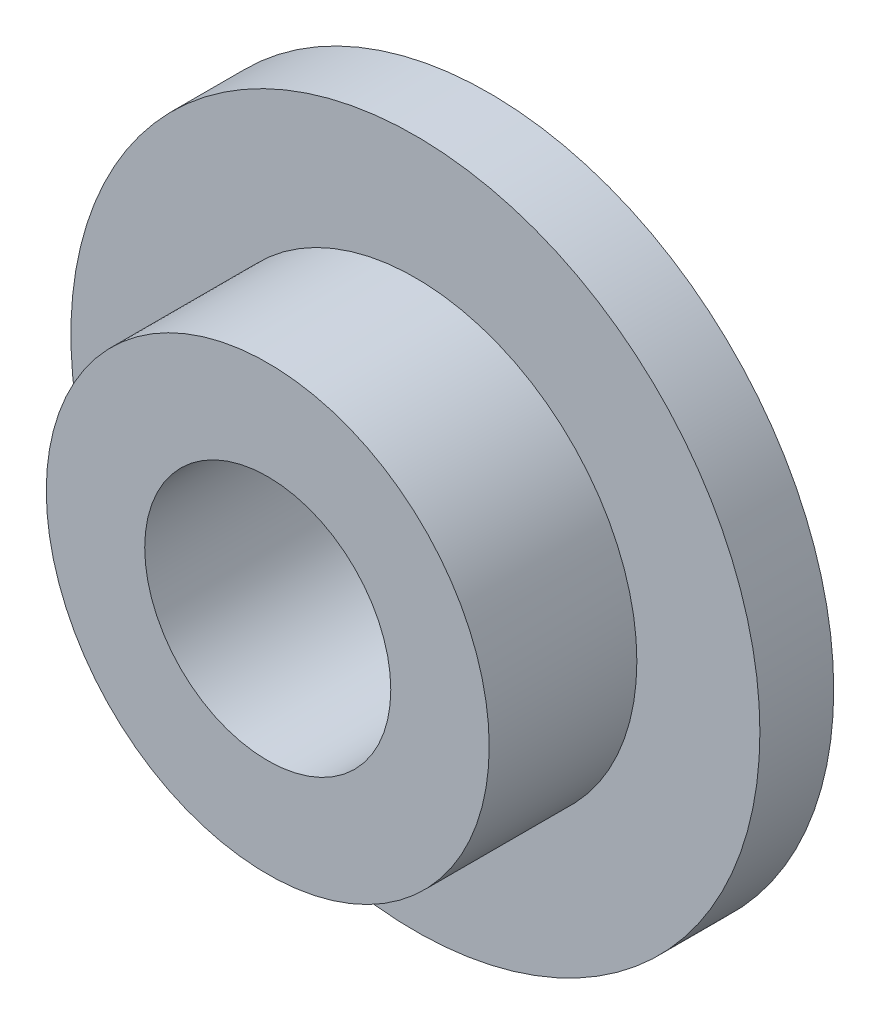
from build123d import *

# Parameters (mm, degrees)
SKETCH1_R           = 14
BOSS_EXTRUDE1_DEPTH = 3
SKETCH2_R           = 9
BOSS_EXTRUDE2_DEPTH = 6
SKETCH3_R           = 5
CUT_EXTRUDE1_DEPTH  = 12


with BuildPart() as part:
    # Sketch1 → Boss-Extrude1 (new body)
    with BuildSketch(Plane.XY):
        Circle(SKETCH1_R)
    extrude(amount=BOSS_EXTRUDE1_DEPTH)

    # Sketch2 → Boss-Extrude2 (add)
    with BuildSketch(Plane.XY.offset(3)):
        Circle(SKETCH2_R)
    extrude(amount=BOSS_EXTRUDE2_DEPTH)

    # Sketch3 → Cut-Extrude1 (cut)
    with BuildSketch(Plane.XY.offset(9)):
        Circle(SKETCH3_R)
    extrude(amount=-CUT_EXTRUDE1_DEPTH, mode=Mode.SUBTRACT)


solid = part.part
